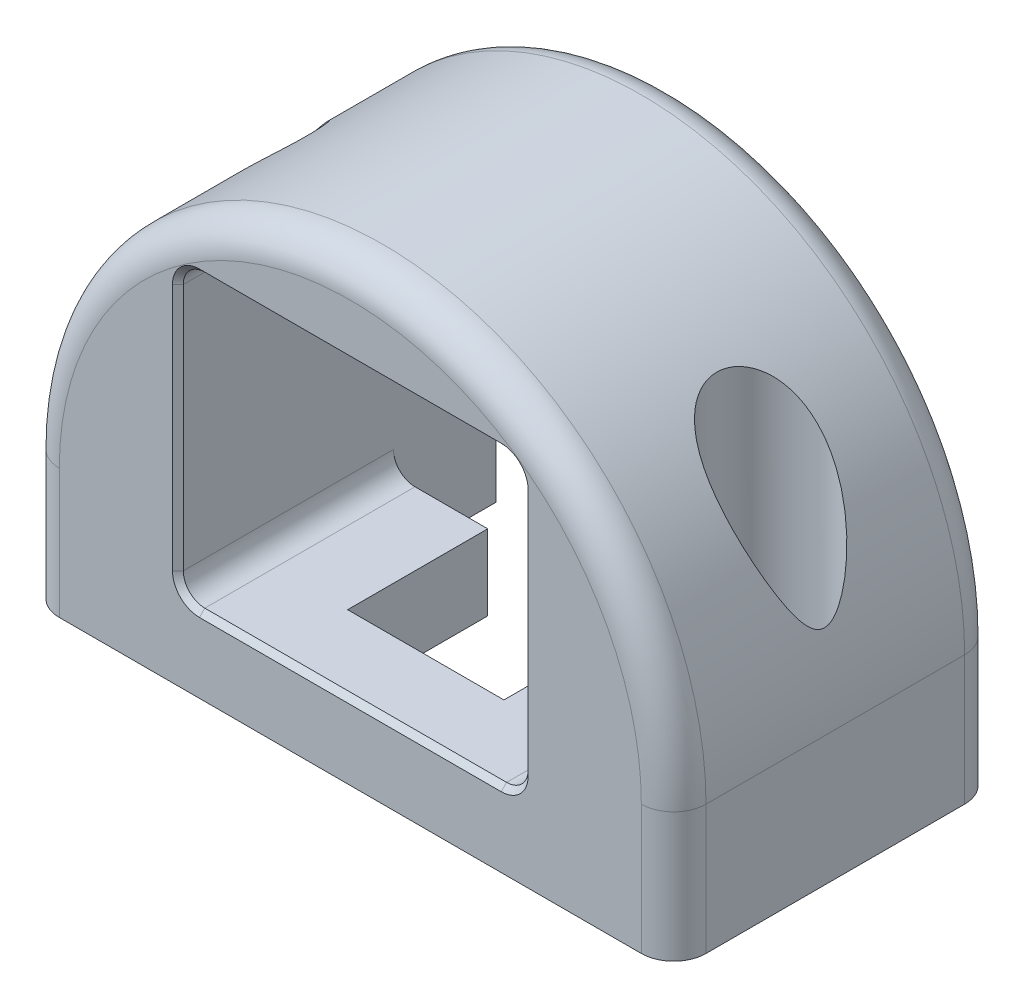
from build123d import *

# Parameters (mm, degrees)
EXTRUDE_1_DEPTH              = 15
HOLE_WIZARD_M5_1_D           = 5.5
HOLE_WIZARD_M5_1_CBORE_D     = 10
HOLE_WIZARD_M5_1_CBORE_DEPTH = 42
SKETCH_4_W                   = 32
SKETCH_4_H                   = 27
CUT_EXTRUDE_2_DEPTH          = 60.699246397
CUT_EXTRUDE_3_DEPTH          = 49.476798739
FILLET_1_R                   = 2
FILLET_2_R                   = 3
CHAMFER_1_SIZE               = 0.5


with BuildPart() as part:
    # 草圖1 → 伸長1 (new, symmetric)
    with BuildSketch(Plane.XY):
        with BuildLine():
            Line((-30, 0), (30, 0))
            Line((30, 0), (30, 12))
            ThreePointArc((30, 12), (0, 42), (-30, 12))
            Line((-30, 12), (-30, 0))
        make_face()
    extrude(amount=EXTRUDE_1_DEPTH, both=True)

    # M5 六角承窩頭蓋螺釘的柱孔1 (through all)
    with Locations(Plane(origin=(0, 50, 0), x_dir=(1, 0, 0), z_dir=(0, 1, 0))):
        with Locations((-24, 0), (24, 0)):
            CounterBoreHole(HOLE_WIZARD_M5_1_D / 2, HOLE_WIZARD_M5_1_CBORE_D / 2, HOLE_WIZARD_M5_1_CBORE_DEPTH)

    # 草圖4 → 伸長2 (cut, through all)
    with BuildSketch(Plane.XY.offset(15)):
        with Locations((0, 20.5)):
            Rectangle(SKETCH_4_W, SKETCH_4_H)
    extrude(amount=-CUT_EXTRUDE_2_DEPTH, mode=Mode.SUBTRACT)

    # 草圖5 → 伸長3 (cut, through all)
    with BuildSketch(Plane(origin=(0, 7, 0), x_dir=(1, 0, 0), z_dir=(0, 1, 0))):
        Polygon((-16, 15), (-16, 5), (-7.25, 5), (-7.25, -8), (7.25, -8), (7.25, 5), (16, 5), (16, 15), align=None)
    extrude(amount=-CUT_EXTRUDE_3_DEPTH, mode=Mode.SUBTRACT)

    # 圓角1
    fillet_1_edges = [part.edges().sort_by_distance(p)[0] for p in [
        (-16, 34, 0),
        (16, 34, 0),
        (16, 7, 5),
        (-16, 7, 5),
    ]]
    fillet(fillet_1_edges, radius=FILLET_1_R)

    # 圓角2
    fillet_2_edges = [part.edges().sort_by_distance(p)[0] for p in [
        (30, 6, 15),
        (0, 42, 15),
        (-30, 6, 15),
        (0, 42, -15),
        (30, 6, -15),
        (-30, 6, -15),
    ]]
    fillet(fillet_2_edges, radius=FILLET_2_R)

    # 導角1
    chamfer_1_edges = [part.edges().sort_by_distance(p)[0] for p in [
        (16, 16, -15),
        (16, 20.5, 15),
        (0, 7, 15),
        (-16, 20.5, 15),
        (-16, 16, -15),
        (0, 34, 15),
        (0, 34, -15),
        (15.414213562, 7.585786438, 15),
        (-15.414213562, 7.585786438, 15),
        (-15.414213562, 33.414213562, 15),
        (-15.414213562, 33.414213562, -15),
        (15.414213562, 33.414213562, 15),
        (15.414213562, 33.414213562, -15),
    ]]
    chamfer(chamfer_1_edges, length=CHAMFER_1_SIZE)


solid = part.part
